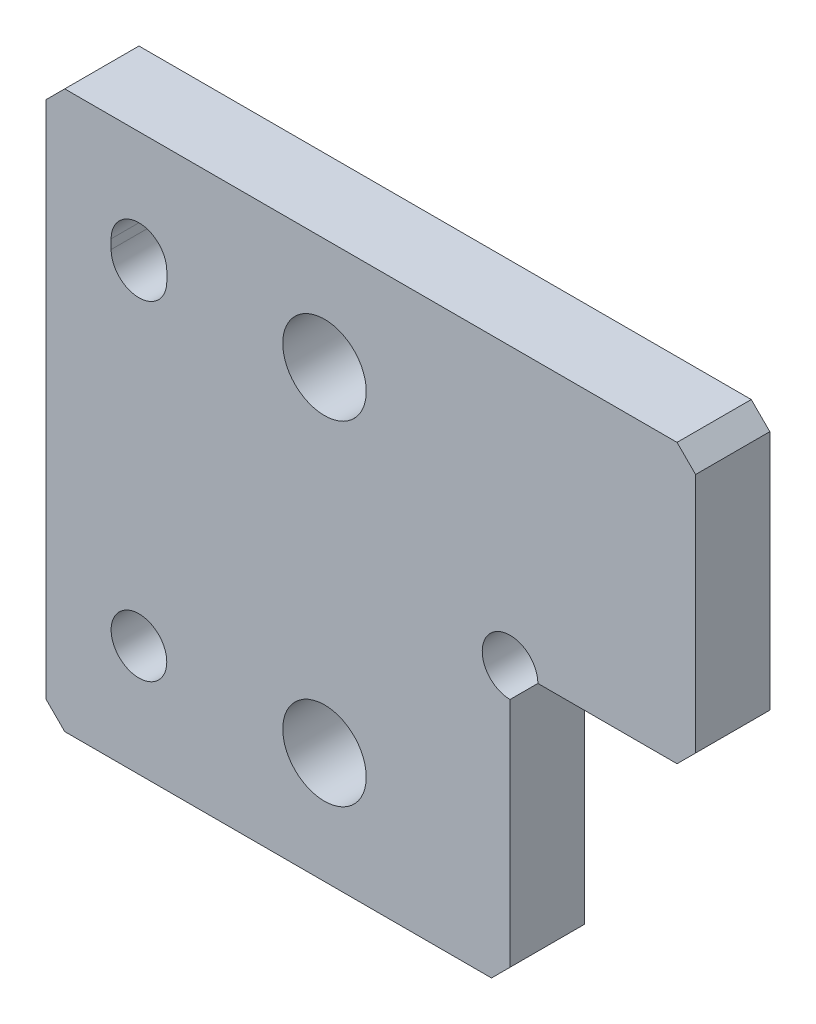
SolidWorks part; units mm, degrees
ref_plane "Front Plane" through (0, 0, 0) normal (0, 0, 1) x (1, 0, 0)
ref_plane "Top Plane" through (0, 0, 0) normal (0, 1, 0) x (1, 0, 0)
ref_plane "Right Plane" through (0, 0, 0) normal (1, 0, 0) x (0, 0, -1)
sketch "Sketch1" plane through (0, 0, 0) normal (0, 0, 1) x (1, 0, 0)
  line L1 (-17.5, 15) -> (17.5, 15)
  line L2 (-17.5, 15) -> (-17.5, -15)
  line L3 (-17.5, -15) -> (17.5, -15)
  line L4 (17.5, 15) -> (17.5, -15)
  line L5 (-17.5, 15) -> (17.5, -15) construction
  line L6 (-17.5, -15) -> (17.5, 15) construction
  point P0 (0, 0)
  dimension "D1" = 35
  dimension "D2" = 30
extrude "Boss-Extrude1" add sketch "Sketch1" along normal mid plane 4
sketch "Sketch2" plane through (0, 0, 2) normal (0, 0, 1) x (1, 0, 0)
  line L0 (-17.5, 15) -> (-17.5, -15) construction
  line L1 (17.5, -15) -> (7.5, -15)
  line L2 (17.5, -15) -> (17.5, 0)
  line L3 (17.5, 0) -> (7.5, 0)
  line L4 (7.5, -15) -> (7.5, 0)
  line L5 (17.5, 15) -> (-17.5, 15) construction
  dimension "D1" = 25
  dimension "D2" = 15
extrude "Cut-Extrude1" cut sketch "Sketch2" against normal through all
hole_wizard "Ø3.0 (3) Diameter Hole2" positions "Sketch4" profile "Sketch3" hole size "Ø3.0" standard "Gb" end condition through all
sketch "Sketch4" plane through (0, 0, 2) normal (0, 0, 1) x (1, 0, 0)
  point P0 (7.5, 0)
sketch "Sketch3" plane through (7.5, 0, 2) normal (1, 0, 0) x (0, -1, 0)
  line L0 (0, 0) -> (0, 4)
  line L1 (0, 4) -> (1.5, 4)
  line L2 (1.5, 4) -> (1.5, 0)
  line L5 (1.5, 0) -> (0, 0)
  line L11 (0, -6.35) -> (0, 107.95) construction
  dimension "通孔孔直径" = 3
  dimension "通孔孔深度" = 4
hole_wizard "Ø3.0 (3) Diameter Hole1" positions "Sketch6" profile "Sketch5" hole size "Ø3.0" standard "Gb" end condition through all
sketch "Sketch6" plane through (0, 0, 2) normal (0, 0, 1) x (1, 0, 0)
  line L0 (0, 0) -> (-25.6795, 0) construction
  line L3 (17.5, 0) -> (17.5, 15) construction
  point P0 (-12.5, 9)
  point P2 (-12.5, -9)
  dimension "D1" = 18
  dimension "D2" = 30
sketch "Sketch5" plane through (-12.5, 9, 2) normal (1, 0, 0) x (0, -1, 0)
  line L0 (0, 0) -> (0, 4)
  line L1 (0, 4) -> (1.5, 4)
  line L2 (1.5, 4) -> (1.5, 0)
  line L5 (1.5, 0) -> (0, 0)
  line L11 (0, -6.35) -> (0, 107.95) construction
  dimension "通孔孔直径" = 3
  dimension "通孔孔深度" = 4
hole_wizard "Ø4.5 (4.5) Diameter Hole1" positions "Sketch8" profile "Sketch7" hole size "Ø4.5" standard "Gb" end condition through all
sketch "Sketch8" plane through (0, 0, 2) normal (0, 0, 1) x (1, 0, 0)
  line L0 (0, 0) -> (-26.8853, 0) construction
  line L4 (17.5, 0) -> (17.5, 15) construction
  point P0 (-2.5, 9)
  point P2 (-2.5, -9)
  dimension "D1" = 18
  dimension "D2" = 20
sketch "Sketch7" plane through (-2.5, 9, 2) normal (1, 0, 0) x (0, -1, 0)
  line L0 (0, 0) -> (0, 4)
  line L1 (0, 4) -> (2.25, 4)
  line L2 (2.25, 4) -> (2.25, 0)
  line L5 (2.25, 0) -> (0, 0)
  line L11 (0, -6.35) -> (0, 107.95) construction
  dimension "通孔孔直径" = 4.5
  dimension "通孔孔深度" = 4
chamfer "Chamfer1" distance 1 angle 45 5 edges at (-17.5, 15, 0) (17.5, 15, 0) (17.5, 0, 0) (7.5, -15, 0) (-17.5, -15, 0)
sketch "Sketch9" plane through (0, 0, 2) normal (0, 0, 1) x (1, 0, 0)
  line L0 (-12.5, 9.25) -> (-12.5, 8.75) construction
  line L1 (-11, 9.25) -> (-11, 8.75)
  line L2 (-14, 9.25) -> (-14, 8.75)
  arc A0 (-11, 9.25) -> (-14, 9.25) centre (-12.5, 9.25) ccw
  arc A1 (-14, 8.75) -> (-11, 8.75) centre (-12.5, 8.75) ccw
  circle A2 centre (-12.5, 9) radius 1.5 construction
  point P2 (-12.5, 9)
  dimension "D1" = 0.5
extrude "Cut-Extrude2" cut sketch "Sketch9" against normal through all
